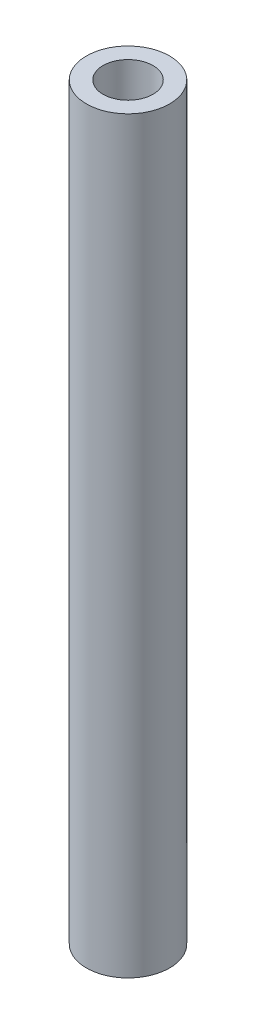
from build123d import *

# Parameters (mm, degrees)
SKETCH1_R           = 2.5
SKETCH1_R_2         = 1.5
BOSS_EXTRUDE1_DEPTH = 45
SKETCH2_R           = 1.5
SKETCH2_R_2         = 0.5
BOSS_EXTRUDE2_DEPTH = 2


with BuildPart() as part:
    # Sketch1 → Boss-Extrude1 (new body)
    with BuildSketch(Plane(origin=(0, 0, 0), x_dir=(1, 0, 0), z_dir=(0, 1, 0))):
        with Locations(Location((0, 0, 0), (0, 0, 90))):
            Circle(SKETCH1_R)
        with Locations(Location((0, 0, 0), (0, 0, 90))):
            Circle(SKETCH1_R_2, mode=Mode.SUBTRACT)
    extrude(amount=BOSS_EXTRUDE1_DEPTH)

    # Sketch2 → Boss-Extrude2 (add)
    with BuildSketch(Plane.XZ):
        with Locations(Location((0, 0, 0), (0, 0, 270))):
            Circle(SKETCH2_R)
        with Locations(Location((0, 0, 0), (0, 0, 270))):
            Circle(SKETCH2_R_2, mode=Mode.SUBTRACT)
    extrude(amount=-BOSS_EXTRUDE2_DEPTH)


solid = part.part
